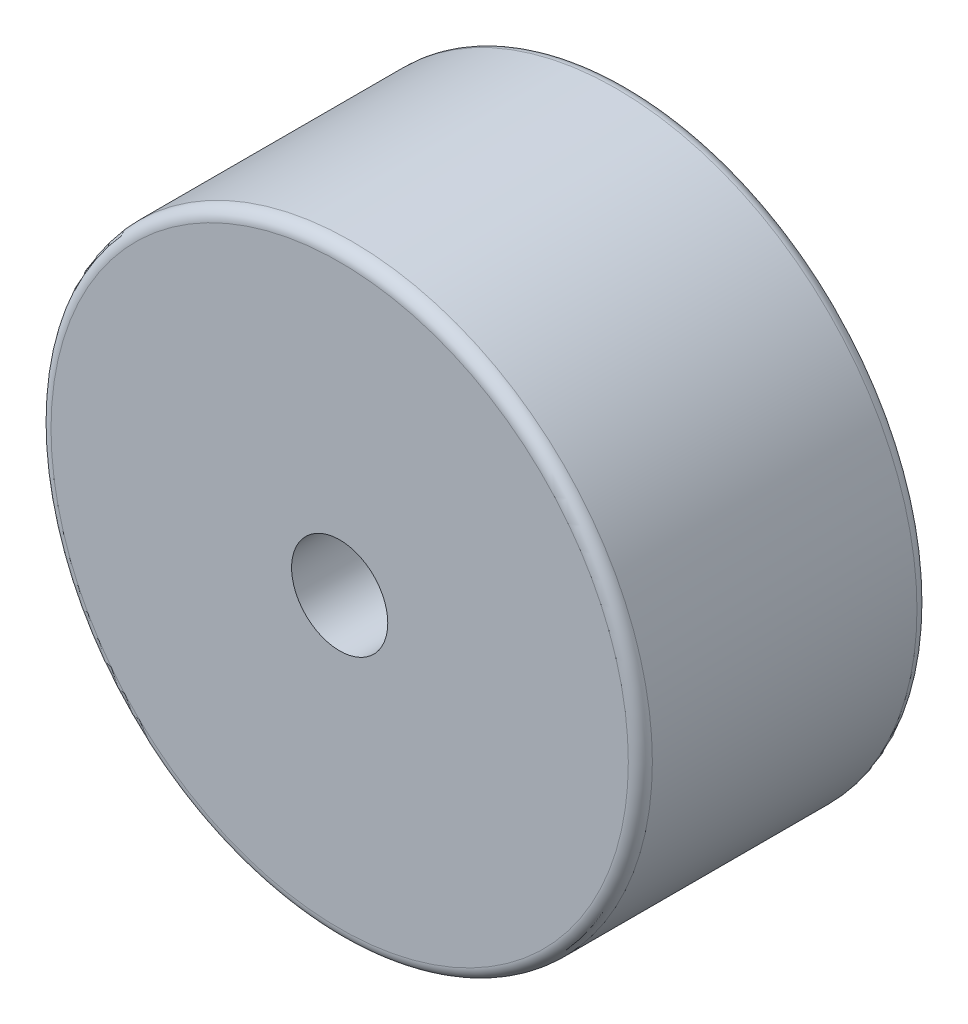
from build123d import *

# Parameters (mm, degrees)
SKETCH_1_R          = 25
EXTRUDE_1_DEPTH     = 24
SKETCH_2_R          = 4
CUT_EXTRUDE_1_DEPTH = 24
FILLET_1_R          = 1


with BuildPart() as part:
    # 草图1 → 凸台-拉伸1 (new body)
    with BuildSketch(Plane.XY):
        Circle(SKETCH_1_R)
    extrude(amount=EXTRUDE_1_DEPTH)

    # 草图2 → 切除-拉伸1 (cut)
    with BuildSketch(Plane.XY.offset(24)):
        Circle(SKETCH_2_R)
    extrude(amount=-CUT_EXTRUDE_1_DEPTH, mode=Mode.SUBTRACT)

    # 圆角1
    fillet_1_edges = [part.edges().sort_by_distance(p)[0] for p in [
        (-25, 0, 0),
        (-25, 0, 24),
    ]]
    fillet(fillet_1_edges, radius=FILLET_1_R)


solid = part.part
